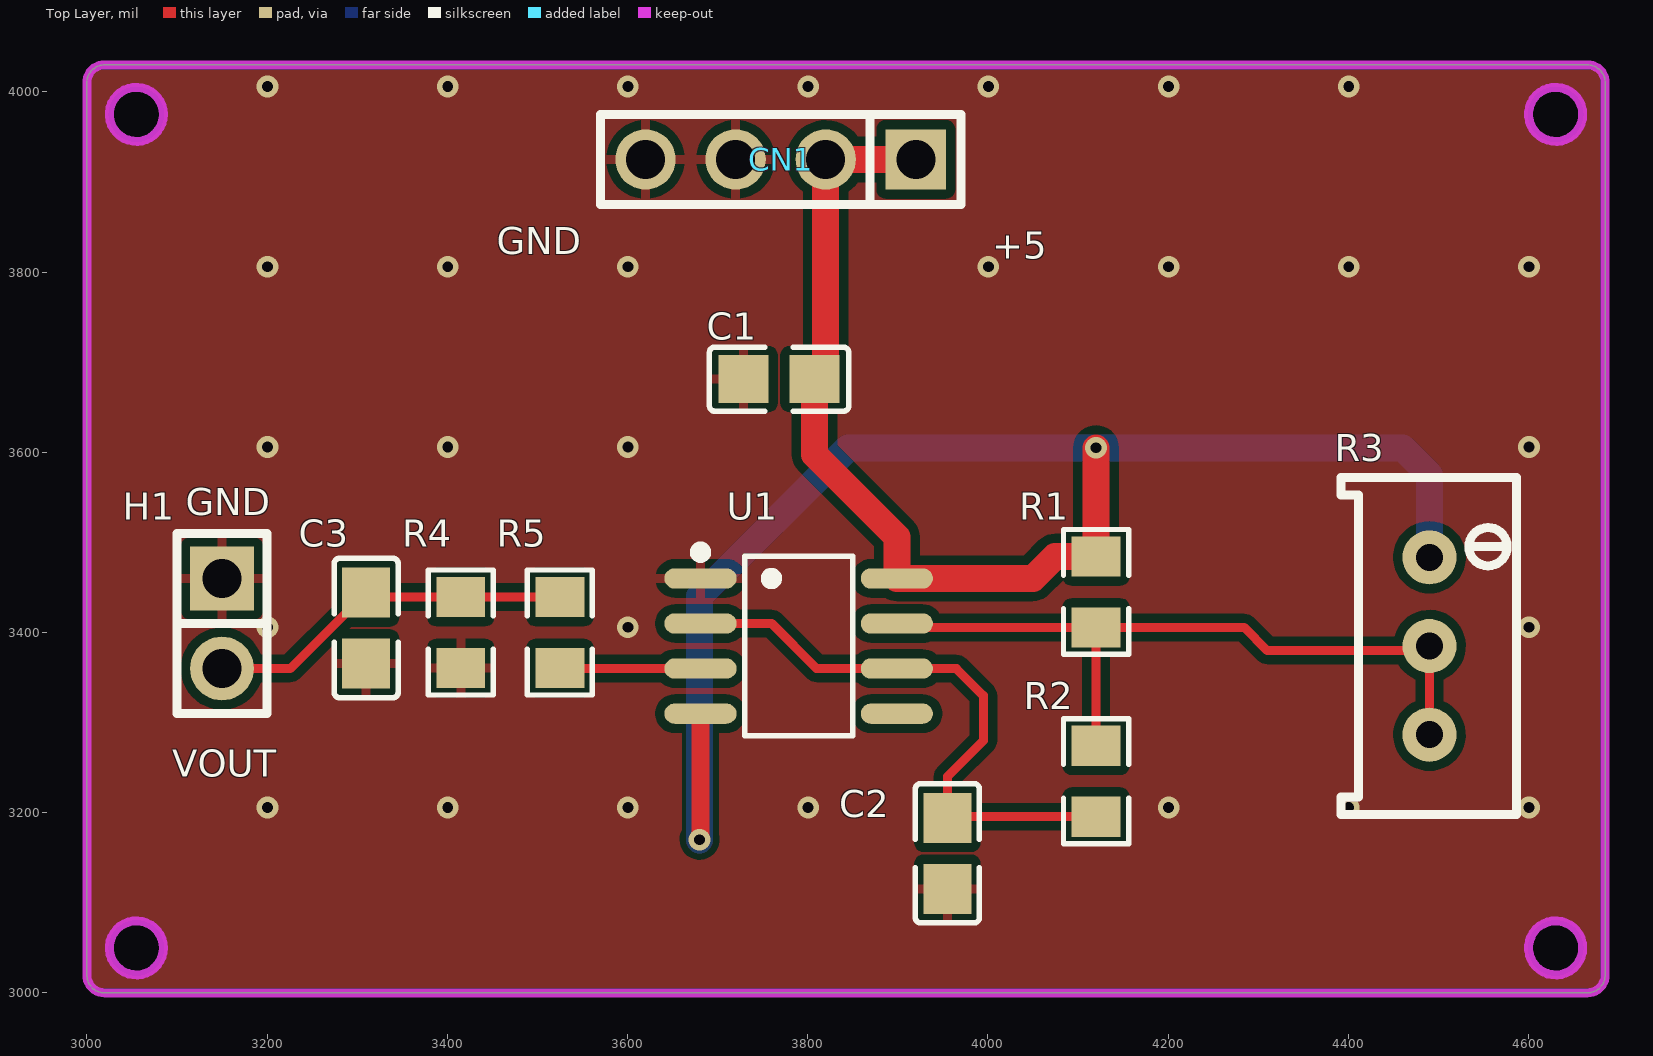
[diagram p0: Top Layer view]
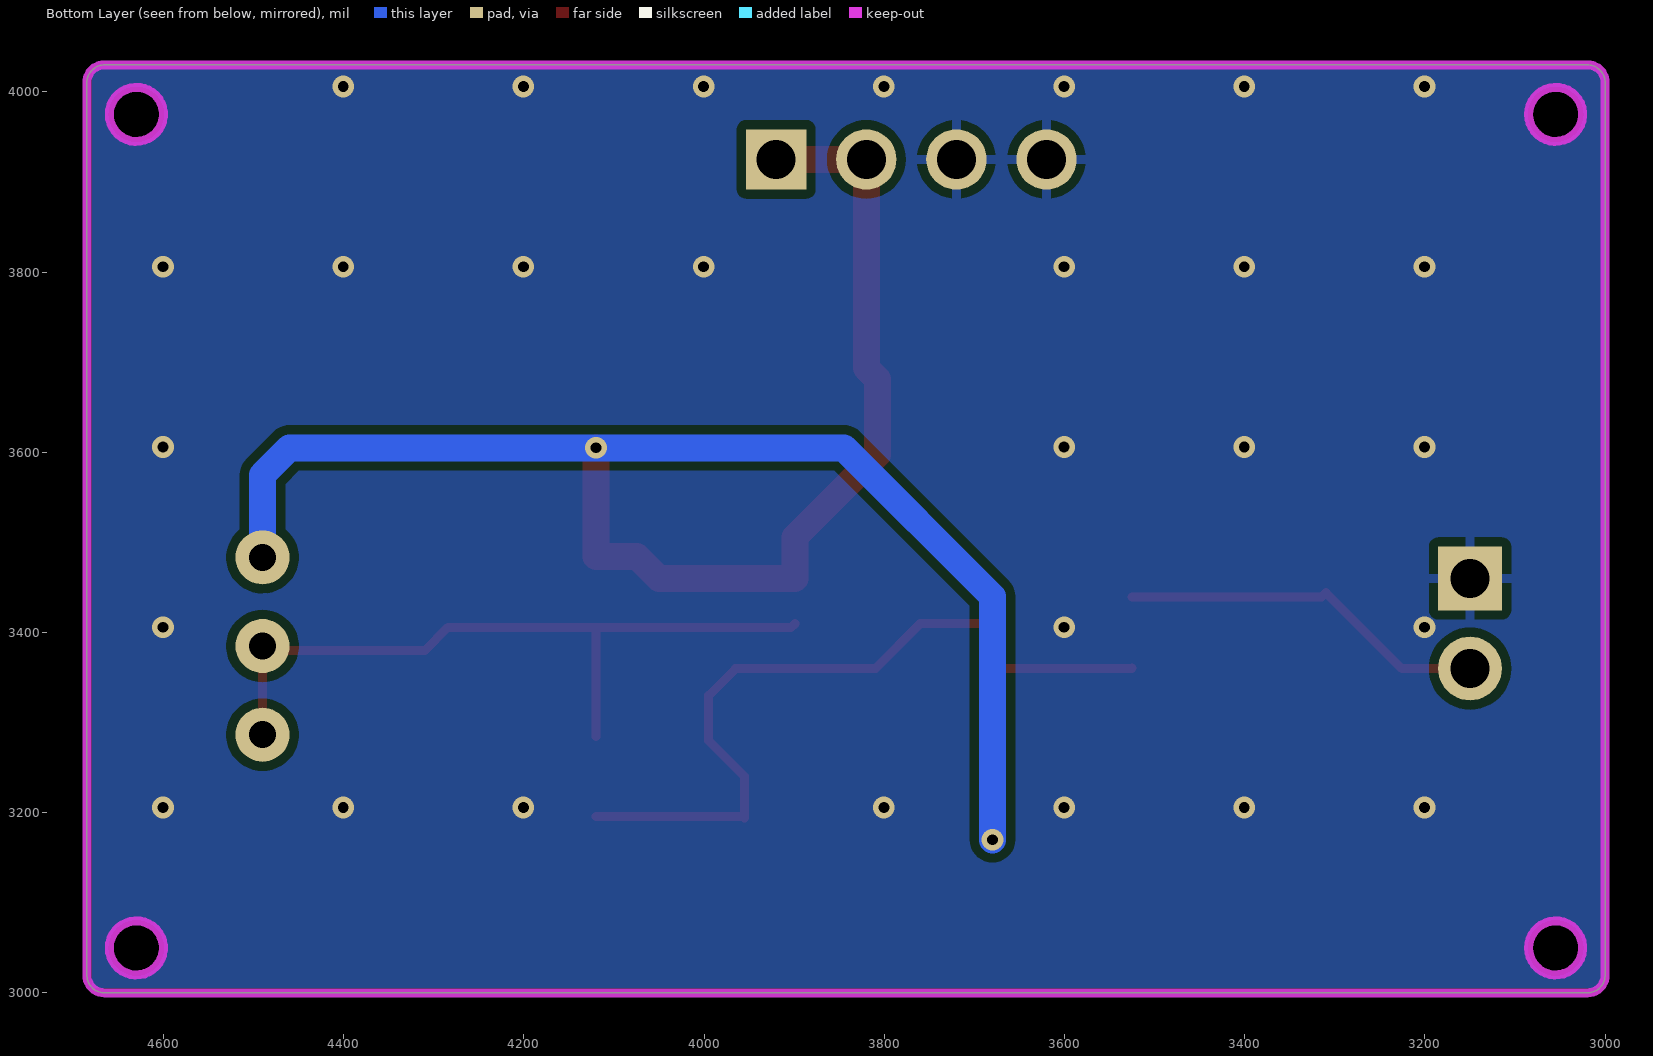
[diagram p1: Bottom Layer view, seen from below]
# Altium PCB MISC89121.pcbdoc
Units mil, origin at the board's own origin, x right, y up, seen from the top; angles counter-clockwise.
Board outline 1685 x 1030 mil, 2 copper layers (Top Layer, Bottom Layer); 11 components, 6 nets, 31 pads, 30 vias.

## Layer stack, top to bottom (the 12.6 mil dielectric is the usual default, probably not edited)
Top Solder Mask Layer: solder mask 0.394, Dk 3.3
Top Layer: signal copper (thickness not stored)
SUBSTRATE1: surface 12.6, FR-4, Dk 4.8
Bottom Layer: signal copper 1.378
Bottom Solder Mask Layer: solder mask 0.394, Dk 3.3

## Board outline
3000,4010 cw(c3020,4010) 3020,4030 4665,4030 cw(c4665,4010) 4685,4010 4685,3020 cw(c4665,3020) 4665,3000 3020,3000 cw(c3020,3020) 3000,3020
cut-out: 3085,3975 3084.63,3979.69 3083.53,3984.27 3081.73,3988.62 3079.27,3992.63 3076.21,3996.21 3072.63,3999.27 3068.62,4001.73 3064.27,4003.53 3059.69,4004.63 3055,4005 3050.31,4004.63 3045.73,4003.53 3041.38,4001.73 3037.37,3999.27 3033.79,3996.21 3030.73,3992.63 3028.27,3988.62 3026.47,3984.27 3025.37,3979.69 3025,3975 3025.37,3970.31 3026.47,3965.73 3028.27,3961.38 3030.73,3957.37 3033.79,3953.79 3037.37,3950.73 3041.38,3948.27 3045.73,3946.47 3050.31,3945.37 3055,3945 3059.69,3945.37 3064.27,3946.47 3068.62,3948.27 3072.63,3950.73 3076.21,3953.79 3079.27,3957.37 3081.73,3961.38 3083.53,3965.73 3084.63,3970.31
cut-out: 3085,3050 3084.63,3054.69 3083.53,3059.27 3081.73,3063.62 3079.27,3067.63 3076.21,3071.21 3072.63,3074.27 3068.62,3076.73 3064.27,3078.53 3059.69,3079.63 3055,3080 3050.31,3079.63 3045.73,3078.53 3041.38,3076.73 3037.37,3074.27 3033.79,3071.21 3030.73,3067.63 3028.27,3063.62 3026.47,3059.27 3025.37,3054.69 3025,3050 3025.37,3045.31 3026.47,3040.73 3028.27,3036.38 3030.73,3032.37 3033.79,3028.79 3037.37,3025.73 3041.38,3023.27 3045.73,3021.47 3050.31,3020.37 3055,3020 3059.69,3020.37 3064.27,3021.47 3068.62,3023.27 3072.63,3025.73 3076.21,3028.79 3079.27,3032.37 3081.73,3036.38 3083.53,3040.73 3084.63,3045.31
cut-out: 4660,3975 4659.63,3979.69 4658.53,3984.27 4656.73,3988.62 4654.27,3992.63 4651.21,3996.21 4647.63,3999.27 4643.62,4001.73 4639.27,4003.53 4634.69,4004.63 4630,4005 4625.31,4004.63 4620.73,4003.53 4616.38,4001.73 4612.37,3999.27 4608.79,3996.21 4605.73,3992.63 4603.27,3988.62 4601.47,3984.27 4600.37,3979.69 4600,3975 4600.37,3970.31 4601.47,3965.73 4603.27,3961.38 4605.73,3957.37 4608.79,3953.79 4612.37,3950.73 4616.38,3948.27 4620.73,3946.47 4625.31,3945.37 4630,3945 4634.69,3945.37 4639.27,3946.47 4643.62,3948.27 4647.63,3950.73 4651.21,3953.79 4654.27,3957.37 4656.73,3961.38 4658.53,3965.73 4659.63,3970.31
cut-out: 4660,3050 4659.63,3054.69 4658.53,3059.27 4656.73,3063.62 4654.27,3067.63 4651.21,3071.21 4647.63,3074.27 4643.62,3076.73 4639.27,3078.53 4634.69,3079.63 4630,3080 4625.31,3079.63 4620.73,3078.53 4616.38,3076.73 4612.37,3074.27 4608.79,3071.21 4605.73,3067.63 4603.27,3063.62 4601.47,3059.27 4600.37,3054.69 4600,3050 4600.37,3045.31 4601.47,3040.73 4603.27,3036.38 4605.73,3032.37 4608.79,3028.79 4612.37,3025.73 4616.38,3023.27 4620.73,3021.47 4625.31,3020.37 4630,3020 4634.69,3020.37 4639.27,3021.47 4643.62,3023.27 4647.63,3025.73 4651.21,3028.79 4654.27,3032.37 4656.73,3036.38 4658.53,3040.73 4659.63,3045.31

## Design rules (kind name [scope] priority, off if disabled: settings)
BoardOutlineClearance copperThickness2oz_1 [All] p2 off: genericclearance=8 ignorepadtopadclearanceinfootprint=FALSE except(0: Arc-SplitContinuation Track-SplitContinuation SMDPad-SplitContinuation THPad-SplitContinuation Via-SplitContinuation Fill-SplitContinuation Region-SplitContinuation Poly-SplitContinuation Text-SplitContinuation Hole-SplitContinuation; 7: Arc-OutlineEdge Track-OutlineEdge SMDPad-OutlineEdge THPad-OutlineEdge Via-OutlineEdge Fill-OutlineEdge Region-OutlineEdge Text-OutlineEdge Hole-OutlineEdge Arc-CutoutEdge Track-CutoutEdge SMDPad-CutoutEdge THPad-CutoutEdge Via-CutoutEdge Fill-CutoutEdge Region-CutoutEdge Text-CutoutEdge Hole-CutoutEdge; 10: Poly-OutlineEdge Poly-CutoutEdge)
BoardOutlineClearance Plane_innerPlane_1 [All] p4 off: genericclearance=4 ignorepadtopadclearanceinfootprint=FALSE except(0: Poly-OutlineEdge Poly-CutoutEdge Arc-SplitContinuation Track-SplitContinuation SMDPad-SplitContinuation THPad-SplitContinuation Via-SplitContinuation Fill-SplitContinuation Region-SplitContinuation Poly-SplitContinuation Text-SplitContinuation Hole-SplitContinuation; 7: Arc-OutlineEdge Track-OutlineEdge SMDPad-OutlineEdge THPad-OutlineEdge Via-OutlineEdge Fill-OutlineEdge Region-OutlineEdge Text-OutlineEdge Hole-OutlineEdge Arc-CutoutEdge Track-CutoutEdge SMDPad-CutoutEdge THPad-CutoutEdge Via-CutoutEdge Fill-CutoutEdge Region-CutoutEdge Text-CutoutEdge Hole-CutoutEdge)
BoardOutlineClearance Copper_copperRegion_1 [All] p6 off: genericclearance=4 ignorepadtopadclearanceinfootprint=FALSE except(0: Poly-OutlineEdge Poly-CutoutEdge Arc-SplitContinuation Track-SplitContinuation SMDPad-SplitContinuation THPad-SplitContinuation Via-SplitContinuation Fill-SplitContinuation Region-SplitContinuation Poly-SplitContinuation Text-SplitContinuation Hole-SplitContinuation; 7: Arc-OutlineEdge Track-OutlineEdge SMDPad-OutlineEdge THPad-OutlineEdge Via-OutlineEdge Fill-OutlineEdge Region-OutlineEdge Text-OutlineEdge Hole-OutlineEdge Arc-CutoutEdge Track-CutoutEdge SMDPad-CutoutEdge THPad-CutoutEdge Via-CutoutEdge Fill-CutoutEdge Region-CutoutEdge Text-CutoutEdge Hole-CutoutEdge)
BoardOutlineClearance copperThickness1oz_1 [All] p8: genericclearance=4 ignorepadtopadclearanceinfootprint=FALSE except(0: Arc-SplitContinuation Track-SplitContinuation SMDPad-SplitContinuation THPad-SplitContinuation Via-SplitContinuation Fill-SplitContinuation Region-SplitContinuation Poly-SplitContinuation Text-SplitContinuation Hole-SplitContinuation; 7: Arc-OutlineEdge Track-OutlineEdge SMDPad-OutlineEdge THPad-OutlineEdge Via-OutlineEdge Fill-OutlineEdge Region-OutlineEdge Text-OutlineEdge Hole-OutlineEdge Arc-CutoutEdge Track-CutoutEdge SMDPad-CutoutEdge THPad-CutoutEdge Via-CutoutEdge Fill-CutoutEdge Region-CutoutEdge Text-CutoutEdge Hole-CutoutEdge; 10: Poly-OutlineEdge Poly-CutoutEdge)
Clearance copperThickness2oz [All] p1 off: gap=8 ignorepadtopadclearanceinfootprint=FALSE except(6: SMDPad-Track SMDPad-SMDPad THPad-Track SMDPad-THPad THPad-THPad Track-Via SMDPad-Via THPad-Via Via-Via Fill-Track Region-Track Fill-SMDPad Region-SMDPad Fill-THPad Region-THPad Fill-Via Region-Via Fill-Fill Fill-Region Region-Region Arc-Track Arc-SMDPad Arc-THPad Arc-Via Fill-Arc Region-Arc Arc-Arc Text-Track SMDPad-Text Text-THPad Text-Via Fill-Text Region-Text Arc-Text Text-Text; 6.9: Hole-Track Hole-SMDPad Hole-THPad Hole-Via Fill-Hole Region-Hole Hole-Arc Hole-Text; 10: Poly-Track Poly-SMDPad Poly-THPad Poly-Via Poly-Fill Poly-Region Poly-Poly Poly-Arc Poly-Text Poly-Hole)
Clearance Plane_innerPlane [All] p3 off: gap=4 ignorepadtopadclearanceinfootprint=FALSE except(6: SMDPad-Track SMDPad-SMDPad THPad-Track SMDPad-THPad THPad-THPad Track-Via SMDPad-Via THPad-Via Via-Via Fill-Track Region-Track Fill-SMDPad Region-SMDPad Fill-THPad Region-THPad Fill-Via Region-Via Fill-Fill Fill-Region Region-Region Poly-Track Poly-SMDPad Poly-THPad Poly-Via Poly-Fill Poly-Region Poly-Poly Arc-Track Arc-SMDPad Arc-THPad Arc-Via Fill-Arc Region-Arc Poly-Arc Arc-Arc Text-Track SMDPad-Text Text-THPad Text-Via Fill-Text Region-Text Poly-Text Arc-Text Text-Text Poly-Hole; 6.9: Hole-Track Hole-SMDPad Hole-THPad Hole-Via Fill-Hole Region-Hole Hole-Arc Hole-Text)
Clearance Copper_copperRegion [All] p5 off: gap=4 ignorepadtopadclearanceinfootprint=FALSE except(6: SMDPad-Track SMDPad-SMDPad THPad-Track SMDPad-THPad THPad-THPad Track-Via SMDPad-Via THPad-Via Via-Via Fill-Track Region-Track Fill-SMDPad Region-SMDPad Fill-THPad Region-THPad Fill-Via Region-Via Fill-Fill Fill-Region Region-Region Arc-Track Arc-SMDPad Arc-THPad Arc-Via Fill-Arc Region-Arc Arc-Arc Text-Track SMDPad-Text Text-THPad Text-Via Fill-Text Region-Text Arc-Text Text-Text; 6.9: Hole-Track Hole-SMDPad Hole-THPad Hole-Via Fill-Hole Region-Hole Hole-Arc Hole-Text; 10: Poly-Track Poly-SMDPad Poly-THPad Poly-Via Poly-Fill Poly-Region Poly-Poly Poly-Arc Poly-Text Poly-Hole)
Clearance copperThickness1oz [All] p7: gap=4 ignorepadtopadclearanceinfootprint=FALSE except(6: SMDPad-Track SMDPad-SMDPad THPad-Track SMDPad-THPad THPad-THPad Track-Via SMDPad-Via THPad-Via Via-Via Fill-Track Region-Track Fill-SMDPad Region-SMDPad Fill-THPad Region-THPad Fill-Via Region-Via Fill-Fill Fill-Region Region-Region Arc-Track Arc-SMDPad Arc-THPad Arc-Via Fill-Arc Region-Arc Arc-Arc Text-Track SMDPad-Text Text-THPad Text-Via Fill-Text Region-Text Arc-Text Text-Text; 6.9: Hole-Track Hole-SMDPad Hole-THPad Hole-Via Fill-Hole Region-Hole Hole-Arc Hole-Text; 10: Poly-Track Poly-SMDPad Poly-THPad Poly-Via Poly-Fill Poly-Region Poly-Poly Poly-Arc Poly-Text Poly-Hole)
DiffPairsRouting differentialPair [All] p1: maxlimit=6 minlimit=0 mostfreqgap=6 toplayer_minwidth=5 toplayer_prefwidth=10 toplayer_maxwidth=100 toplayer_mingap=0 toplayer_prefgap=6 toplayer_maxgap=6 bottomlayer_minwidth=5 bottomlayer_prefwidth=10 bottomlayer_maxwidth=100 bottomlayer_mingap=0 bottomlayer_prefgap=6 bottomlayer_maxgap=6 maxuncoupledlength=10
HoleToHoleClearance otherClearance [All] p1: gap=11.81 allowstackedmicrovias=TRUE
Length netLength [All] p1: minlimit=0 maxlimit=0
PasteMaskExpansion pasteMaskExpansion [All] p1: expansion=0
PlaneConnect innerPlane [All] p1: planeconnectstyle=Relief reliefexpansion=20 reliefentries=4 reliefconductorwidth=10 reliefairgap=10
PolygonConnect copperRegion [All] p1: connectstyle=Relief reliefconductorwidth=10 reliefentries=4 polygonreliefangle="90 Angle" airgapwidth=10 via.connectstyle=Relief via.reliefconductorwidth=10 via.reliefentries=4 via.polygonreliefangle="90 Angle" via.airgapwidth=10
RoutingVias viaSize [All] p1: holewidth=12.01 width=24.02 viastyle="Through Hole" minholewidth=11.81 minwidth=19.68 maxholewidth=248.03 maxwidth=393.7
SolderMaskExpansion solderMaskExpansion [All] p1: expansion=2 istentingtop=FALSE
Width copperThickness2oz_2 [All] p1 off: maxlimit=100 minlimit=8 preferedwidth=10
Width copperThickness1oz_2 [All] p2: maxlimit=100 minlimit=5 preferedwidth=10

## Components (designator, comment, footprint, x,y, rotation, side; value= is the part's Value field where it differs from the comment)
C1 "1uF" C0805 3768.21,3681.15 r0 top
C2 "10nF" C0805 3955,3155 r90 top
C3 "200pF" C0805 3310,3405 r90 top
CN1 "A2541WV-4P" HDR-TH_4P-P2.54-V-M 3770,3925 r180 top
H1 "A2541WV-2P" HDR-TH_P2.54-H-M_A2541WV-2P 3150,3410 r270 top
R1 "5kΩ" R0805 4120,3445 r90 top
R2 "3kΩ" R0805 4120,3235 r90 top
R3 "5kΩ" RES-ADJ-TH_3P-L10.0-W10.0-P2.50-L 4490,3385 r270 top
R4 "10kΩ" R0805 3415,3400 r90 top
R5 "10kΩ" R0805 3525,3400 r270 top
U1 "100kHz" SOP-8_L5.0-W4.0-P1.27-LS6.0-BL 3790,3385 r270 top

## Footprints (in the part's own frame and the unit in brackets; to place one, negate y for a bottom-side part, rotate by r counter-clockwise, add the part's x,y. Pads: shape width x height; smd on the part's side, far side on the other; paste and mask are expansions set on the pad)
C0805 [mm]
  rect 1.41x1.35 smd paste-100 mask+0.051: 1(-1,0) 2(1,0)
  silkscreen extent -1.96,-0.9 1.96,0.9
HDR-TH_4P-P2.54-V-M [mm]
  rect 1.7x1.7 hole 1.1: 1(-3.81,0)
  round 1.7 hole 1.1: 2(-1.27,0) 3(1.27,0) 4(3.81,0)
  silkscreen extent -5.08,-1.27 5.08,1.27
HDR-TH_P2.54-H-M_A2541WV-2P [mm]
  rect 1.8x1.8 hole 1.1: 1(-1.27,0)
  round 1.8 hole 1.1: 2(1.27,0)
  silkscreen extent -2.54,-1.27 2.54,1.27
R0805 [mm]
  rect 1.133x1.377 smd paste-100 mask+0.051: 1(-1,0) 2(1,0)
  silkscreen extent -1.76,-0.92 1.76,0.92
RES-ADJ-TH_3P-L10.0-W10.0-P2.50-L [mil]
  round 60 hole 30: 1(-98.43,0) 2(0.01,0.01) 3(98.43,0)
  silkscreen extent -187,-98 187,96
SOP-8_L5.0-W4.0-P1.27-LS6.0-BL [mil]
  oval 22.6x80.14 smd: 1(-75,-108.97) 2(-25,-108.97) 3(25,-108.97) 4(75,-108.97) 5(75,108.97) 6(25,108.97) 7(-25,108.97) 8(-75,108.97)
  silkscreen extent -110,-115 99,60

## Via types
v1: diameter 24.02, hole 12, Top Layer to Bottom Layer, 30 vias

## Nets (pads, with @x,y where several pads share a name; then routed paths per layer and width w, separated by ;. In a path a pad name is that pad's centre, name@x,y a point inside that pad or via, vN(x,y) a via of type N, cw(c..) or ccw(c..) an arc to the next point about the centre after c; other vN are vias at no path point)
$1N3: R1.1 R2.2 R3.2 R3.3 U1.7 | length 825.2
  Top Layer w10: U1.7 3903.34,3405.63 R1.1 ; R2.2@4120,3284.37 R1.1 ; R3.3 R3.2 4485.01,3380 4310,3380 4284.37,3405.63 R1.1
$1N4: C2.2 R2.1 U1.2 U1.6 | length 664.8
  Top Layer w10: U1.2 3760,3410 3810,3360 U1.6 3965,3360 3995,3330 3995,3280 3955,3240 C2.2 3956.26,3195.63 R2.1
$1N10: C3.2 H1.2 R4.2 R5.1 | length 412
  Top Layer w10: H1.2 3225.63,3360 C3.2 3315,3439.37 R4.2 R5.1
+5V: C1.2 CN1.1 CN1.2 R1.2 R3.1 U1.4 U1.8 | length 2352.5
  Top Layer w20: v1(3680,3170) 3681.03,3171.03 U1.4
  Top Layer w30: CN1.1 CN1.2 3820,3693.57 C1.2 3807.58,3597.42 3898.97,3506.03 U1.8 4050,3460 4074.37,3484.37 R1.2 v1(4120,3605)
  Bottom Layer w30: v1(3680,3170) 3680,3440 3845,3605 v1(4120,3605) 4460,3605 4490,3575 R3.1
GND: C1.1 C2.1 C3.1 CN1.3 CN1.4 H1.1 R4.1 U1.1
  other v1: 3200.5,3205.86 3400.5,3205.86 3600.5,3205.86 3800.5,3205.86 4200.5,3205.86 4400.5,3205.86 4600.5,3205.86 3200.5,3405.86 3600.5,3405.86 4600.5,3405.86 3200.5,3605.86 3400.5,3605.86 3600.5,3605.86 4600.5,3605.86 3200.5,3805.86 3400.5,3805.86 3600.5,3805.86 4000.5,3805.86 4200.5,3805.86 4400.5,3805.86 4600.5,3805.86 3200.5,4005.86 3400.5,4005.86 3600.5,4005.86 3800.5,4005.86 4000.5,4005.86 4200.5,4005.86 4400.5,4005.86
VOUT: R5.2 U1.3 | length 156.3
  Top Layer w10: R5.2 3525.63,3360 U1.3
pads on no net: U1.5

## Polygon pours and split planes (outlines as drawn)
GND on Top Layer (solid, remove dead copper, pour order 0): 3000,3005.86 4679.14,3005.86 4679.14,4024.14 3000,4024.14
GND on Bottom Layer (solid, remove dead copper, pour order 2): 3000,3005.86 4679.14,3005.86 4679.14,4030 3000,4030

## Keep-outs
Board Outline Layer:
  circle w10: c3055,3975 r30
  circle w10: c3055,3050 r30
  circle w10: c4630,3975 r30
  circle w10: c4630,3050 r30
  region: 3085,3975 3084.63,3979.69 3083.53,3984.27 3081.73,3988.62 3079.27,3992.63 3076.21,3996.21 3072.63,3999.27 3068.62,4001.73 3064.27,4003.53 3059.69,4004.63 3055,4005 3050.31,4004.63 3045.73,4003.53 3041.38,4001.73 3037.37,3999.27 3033.79,3996.21 3030.73,3992.63 3028.27,3988.62 3026.47,3984.27 3025.37,3979.69 3025,3975 3025.37,3970.31 3026.47,3965.73 3028.27,3961.38 3030.73,3957.37 3033.79,3953.79 3037.37,3950.73 3041.38,3948.27 3045.73,3946.47 3050.31,3945.37 3055,3945 3059.69,3945.37 3064.27,3946.47 3068.62,3948.27 3072.63,3950.73 3076.21,3953.79 3079.27,3957.37 3081.73,3961.38 3083.53,3965.73 3084.63,3970.31
  region: 3085,3975 3084.63,3979.69 3083.53,3984.27 3081.73,3988.62 3079.27,3992.63 3076.21,3996.21 3072.63,3999.27 3068.62,4001.73 3064.27,4003.53 3059.69,4004.63 3055,4005 3050.31,4004.63 3045.73,4003.53 3041.38,4001.73 3037.37,3999.27 3033.79,3996.21 3030.73,3992.63 3028.27,3988.62 3026.47,3984.27 3025.37,3979.69 3025,3975 3025.37,3970.31 3026.47,3965.73 3028.27,3961.38 3030.73,3957.37 3033.79,3953.79 3037.37,3950.73 3041.38,3948.27 3045.73,3946.47 3050.31,3945.37 3055,3945 3059.69,3945.37 3064.27,3946.47 3068.62,3948.27 3072.63,3950.73 3076.21,3953.79 3079.27,3957.37 3081.73,3961.38 3083.53,3965.73 3084.63,3970.31
  region: 3085,3050 3084.63,3054.69 3083.53,3059.27 3081.73,3063.62 3079.27,3067.63 3076.21,3071.21 3072.63,3074.27 3068.62,3076.73 3064.27,3078.53 3059.69,3079.63 3055,3080 3050.31,3079.63 3045.73,3078.53 3041.38,3076.73 3037.37,3074.27 3033.79,3071.21 3030.73,3067.63 3028.27,3063.62 3026.47,3059.27 3025.37,3054.69 3025,3050 3025.37,3045.31 3026.47,3040.73 3028.27,3036.38 3030.73,3032.37 3033.79,3028.79 3037.37,3025.73 3041.38,3023.27 3045.73,3021.47 3050.31,3020.37 3055,3020 3059.69,3020.37 3064.27,3021.47 3068.62,3023.27 3072.63,3025.73 3076.21,3028.79 3079.27,3032.37 3081.73,3036.38 3083.53,3040.73 3084.63,3045.31
  region: 3085,3050 3084.63,3054.69 3083.53,3059.27 3081.73,3063.62 3079.27,3067.63 3076.21,3071.21 3072.63,3074.27 3068.62,3076.73 3064.27,3078.53 3059.69,3079.63 3055,3080 3050.31,3079.63 3045.73,3078.53 3041.38,3076.73 3037.37,3074.27 3033.79,3071.21 3030.73,3067.63 3028.27,3063.62 3026.47,3059.27 3025.37,3054.69 3025,3050 3025.37,3045.31 3026.47,3040.73 3028.27,3036.38 3030.73,3032.37 3033.79,3028.79 3037.37,3025.73 3041.38,3023.27 3045.73,3021.47 3050.31,3020.37 3055,3020 3059.69,3020.37 3064.27,3021.47 3068.62,3023.27 3072.63,3025.73 3076.21,3028.79 3079.27,3032.37 3081.73,3036.38 3083.53,3040.73 3084.63,3045.31
  region: 4660,3975 4659.63,3979.69 4658.53,3984.27 4656.73,3988.62 4654.27,3992.63 4651.21,3996.21 4647.63,3999.27 4643.62,4001.73 4639.27,4003.53 4634.69,4004.63 4630,4005 4625.31,4004.63 4620.73,4003.53 4616.38,4001.73 4612.37,3999.27 4608.79,3996.21 4605.73,3992.63 4603.27,3988.62 4601.47,3984.27 4600.37,3979.69 4600,3975 4600.37,3970.31 4601.47,3965.73 4603.27,3961.38 4605.73,3957.37 4608.79,3953.79 4612.37,3950.73 4616.38,3948.27 4620.73,3946.47 4625.31,3945.37 4630,3945 4634.69,3945.37 4639.27,3946.47 4643.62,3948.27 4647.63,3950.73 4651.21,3953.79 4654.27,3957.37 4656.73,3961.38 4658.53,3965.73 4659.63,3970.31
  region: 4660,3975 4659.63,3979.69 4658.53,3984.27 4656.73,3988.62 4654.27,3992.63 4651.21,3996.21 4647.63,3999.27 4643.62,4001.73 4639.27,4003.53 4634.69,4004.63 4630,4005 4625.31,4004.63 4620.73,4003.53 4616.38,4001.73 4612.37,3999.27 4608.79,3996.21 4605.73,3992.63 4603.27,3988.62 4601.47,3984.27 4600.37,3979.69 4600,3975 4600.37,3970.31 4601.47,3965.73 4603.27,3961.38 4605.73,3957.37 4608.79,3953.79 4612.37,3950.73 4616.38,3948.27 4620.73,3946.47 4625.31,3945.37 4630,3945 4634.69,3945.37 4639.27,3946.47 4643.62,3948.27 4647.63,3950.73 4651.21,3953.79 4654.27,3957.37 4656.73,3961.38 4658.53,3965.73 4659.63,3970.31
  region: 4660,3050 4659.63,3054.69 4658.53,3059.27 4656.73,3063.62 4654.27,3067.63 4651.21,3071.21 4647.63,3074.27 4643.62,3076.73 4639.27,3078.53 4634.69,3079.63 4630,3080 4625.31,3079.63 4620.73,3078.53 4616.38,3076.73 4612.37,3074.27 4608.79,3071.21 4605.73,3067.63 4603.27,3063.62 4601.47,3059.27 4600.37,3054.69 4600,3050 4600.37,3045.31 4601.47,3040.73 4603.27,3036.38 4605.73,3032.37 4608.79,3028.79 4612.37,3025.73 4616.38,3023.27 4620.73,3021.47 4625.31,3020.37 4630,3020 4634.69,3020.37 4639.27,3021.47 4643.62,3023.27 4647.63,3025.73 4651.21,3028.79 4654.27,3032.37 4656.73,3036.38 4658.53,3040.73 4659.63,3045.31
  region: 4660,3050 4659.63,3054.69 4658.53,3059.27 4656.73,3063.62 4654.27,3067.63 4651.21,3071.21 4647.63,3074.27 4643.62,3076.73 4639.27,3078.53 4634.69,3079.63 4630,3080 4625.31,3079.63 4620.73,3078.53 4616.38,3076.73 4612.37,3074.27 4608.79,3071.21 4605.73,3067.63 4603.27,3063.62 4601.47,3059.27 4600.37,3054.69 4600,3050 4600.37,3045.31 4601.47,3040.73 4603.27,3036.38 4605.73,3032.37 4608.79,3028.79 4612.37,3025.73 4616.38,3023.27 4620.73,3021.47 4625.31,3020.37 4630,3020 4634.69,3020.37 4639.27,3021.47 4643.62,3023.27 4647.63,3025.73 4651.21,3028.79 4654.27,3032.37 4656.73,3036.38 4658.53,3040.73 4659.63,3045.31
  lines w0.1: 3025,3050 cw(c3055,3050) 3085,3050 cw(c3055,3050) 3025,3050 ; 3025,3975 cw(c3055,3975) 3085,3975 cw(c3055,3975) 3025,3975 ; 4600,3050 cw(c4630,3050) 4660,3050 cw(c4630,3050) 4600,3050 ; 4600,3975 cw(c4630,3975) 4660,3975 cw(c4630,3975) 4600,3975
  lines w10: 3000,3020 ccw(c3020,3020) 3020,3000 4665,3000 ccw(c4665,3020) 4685,3020 4685,4010 ccw(c4665,4010) 4665,4030 3020,4030 ccw(c3020,4010) 3000,4010 3000,3020

## Silkscreen, mask and mechanical layers (free items; w line width, h text height)
Top Silkscreen Layer:
  text "GND" at 3455,3820 h30
  text "+5" at 4005,3815 h30
  text "GND" at 3110,3530 h30
  text "VOUT" at 3095,3240 h30
Mechanical Layer:
  circle w1: c3055,3975 r30
  circle w1: c3055,3050 r30
  circle w1: c4630,3975 r30
  circle w1: c4630,3050 r30
  lines w0.1: 3025,3050 cw(c3055,3050) 3085,3050 cw(c3055,3050) 3025,3050 ; 3025,3975 cw(c3055,3975) 3085,3975 cw(c3055,3975) 3025,3975 ; 4600,3050 cw(c4630,3050) 4660,3050 cw(c4630,3050) 4600,3050 ; 4600,3975 cw(c4630,3975) 4660,3975 cw(c4630,3975) 4600,3975